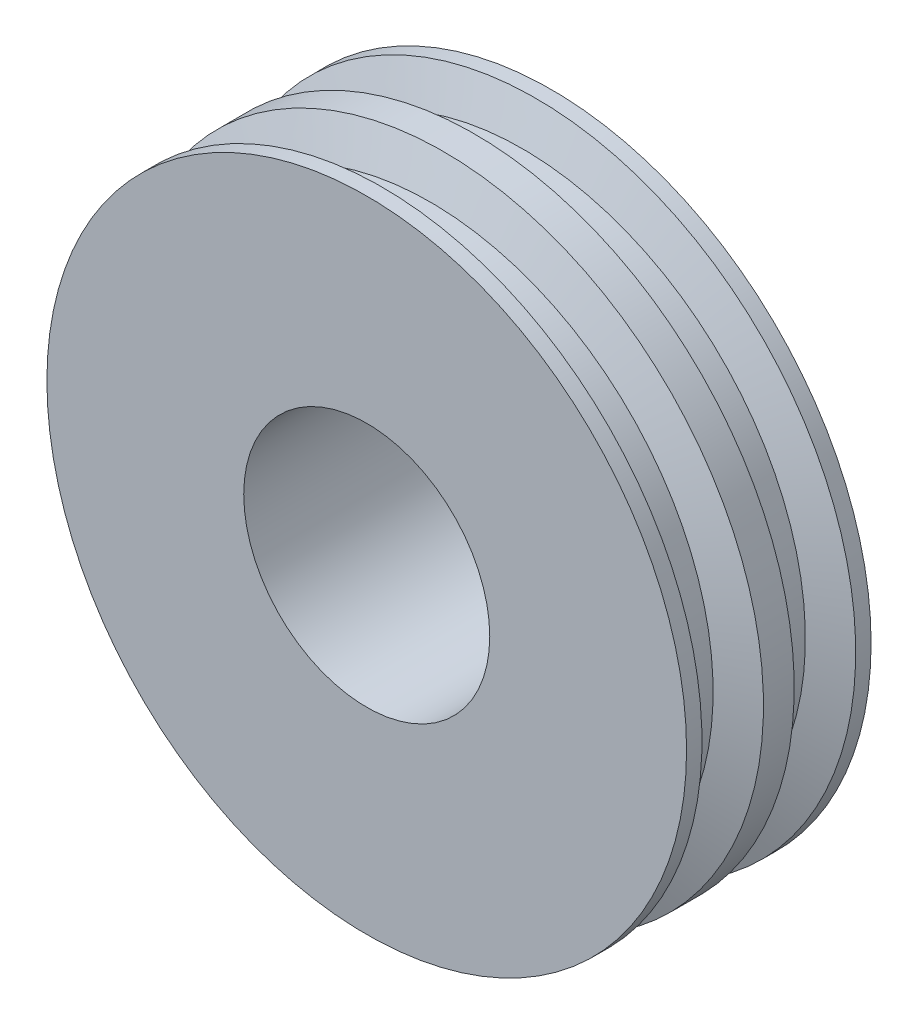
from build123d import *

# Parameters (mm, degrees)
SKETCH1_R           = 52
SKETCH1_R_2         = 20
BOSS_EXTRUDE1_DEPTH = 30


with BuildPart() as part:
    # Sketch1 → Boss-Extrude1 (new body)
    with BuildSketch(Plane.XY):
        Circle(SKETCH1_R)
        Circle(SKETCH1_R_2, mode=Mode.SUBTRACT)
    extrude(amount=BOSS_EXTRUDE1_DEPTH)

    # Sketch2 → Cut-Revolve1 (revolve, cut)
    with BuildSketch(Plane(origin=(0, 0, 0), x_dir=(0, 0, -1), z_dir=(1, 0, 0)), mode=Mode.PRIVATE) as cut_revolve1_sk:
        Polygon((-25.316178594, 46), (-19.683821406, 46), (-17.5, 52), (-27.5, 52), align=None)
        Polygon((-12.5, 52), (-10.316178594, 46), (-4.683821406, 46), (-2.5, 52), align=None)
    revolve(cut_revolve1_sk.sketch.rotate(Axis((0, 0, 0), (0, 0, 1)), 90), axis=Axis((0, 0, 0), (0, 0, 1)), mode=Mode.SUBTRACT)


solid = part.part
